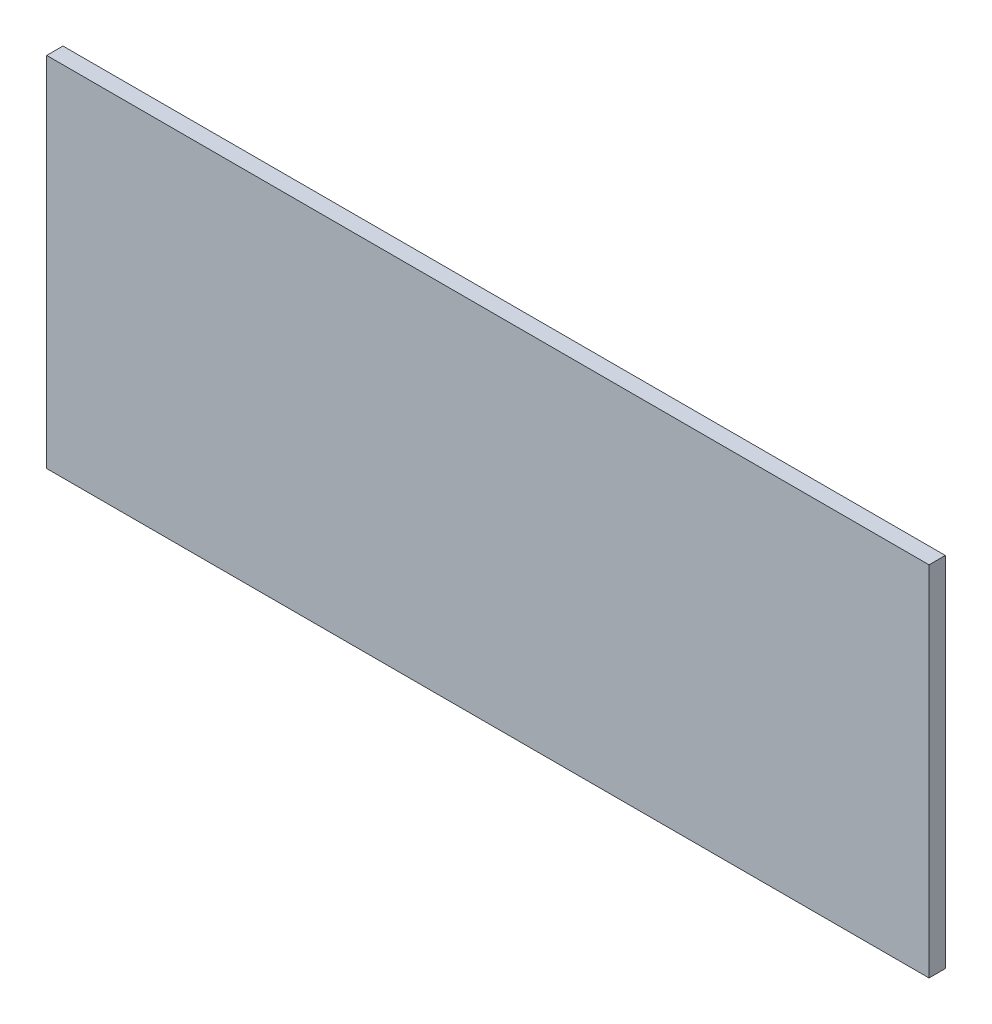
SolidWorks part; units mm, degrees
material "1023 碳钢板 (SS)"
ref_plane "前视基准面" through (0, 0, 0) normal (0, 0, 1) x (1, 0, 0)
ref_plane "上视基准面" through (0, 0, 0) normal (0, 1, 0) x (1, 0, 0)
ref_plane "右视基准面" through (0, 0, 0) normal (1, 0, 0) x (0, 0, -1)
sketch "草图1" plane through (0, 0, 0) normal (0, 0, 1) x (1, 0, 0)
  line L1 (108.5, 44) -> (-108.5, 44)
  line L2 (108.5, 44) -> (108.5, -44)
  line L3 (108.5, -44) -> (-108.5, -44)
  line L4 (-108.5, 44) -> (-108.5, -44)
  line L5 (108.5, 44) -> (-108.5, -44) construction
  line L6 (108.5, -44) -> (-108.5, 44) construction
  point P0 (0, 0)
  dimension "D1" = 217
  dimension "D2" = 88
extrude "凸台-拉伸1" add sketch "草图1" along normal blind 4
